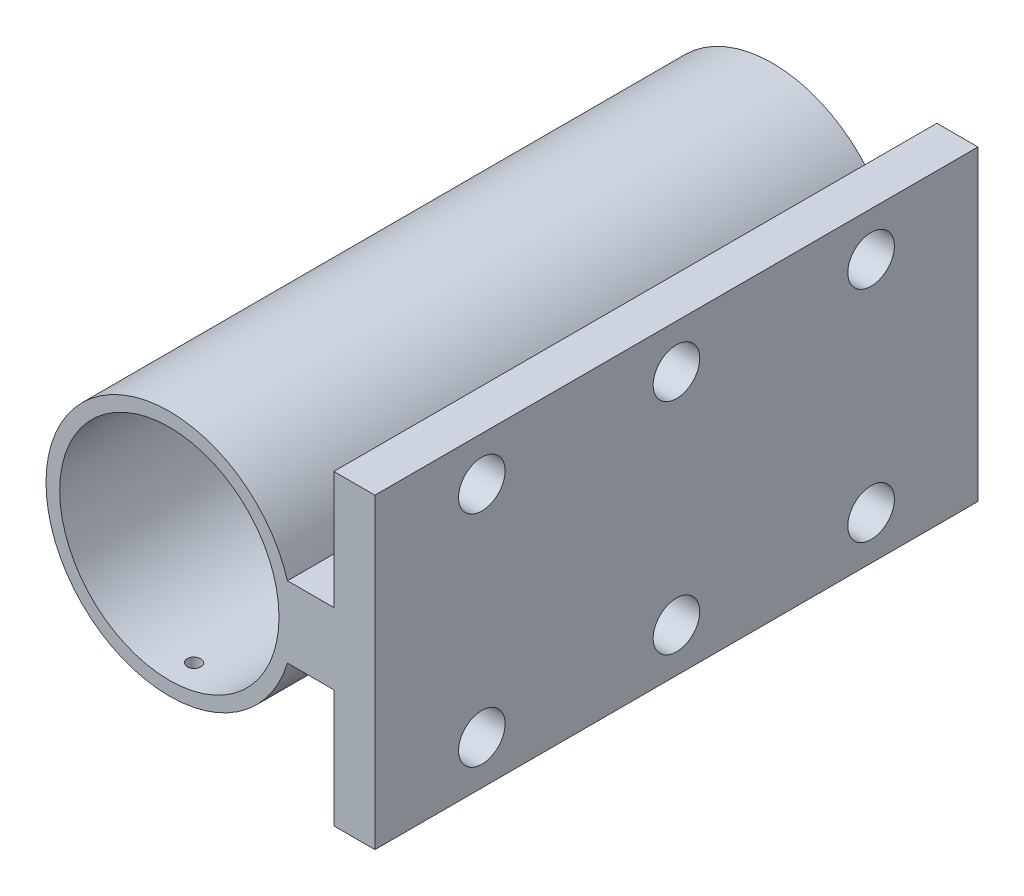
SolidWorks part; units mm, degrees
ref_plane "Front Plane" through (0, 0, 0) normal (0, 0, 1) x (1, 0, 0)
ref_plane "Top Plane" through (0, 0, 0) normal (0, 1, 0) x (1, 0, 0)
ref_plane "Right Plane" through (0, 0, 0) normal (1, 0, 0) x (0, 0, -1)
other "Configuration Table"
sketch "Sketch1" plane through (0, 0, 0) normal (0, 0, 1) x (1, 0, 0)
  line L0 (0, 0) -> (201.2265, 0) construction
  line L2 (75, 56) -> (60, 56)
  line L3 (75, 56) -> (75, -56)
  line L4 (75, -56) -> (60, -56)
  line L5 (60, 56) -> (60, 13)
  line L6 (75, 56) -> (60, -56) construction
  line L7 (75, -56) -> (60, 56) construction
  line L8 (43.0813, -13) -> (60, -13)
  line L10 (60, -13) -> (60, -56)
  line L11 (43.0813, 13) -> (60, 13)
  circle A0 centre (0, 0) radius 40
  arc A1 (43.0813, 13) -> (43.0813, -13) centre (0, 0) ccw
  point P5 (67.5, 0)
  dimension "D1" = 80
  dimension "D2" = 90
  dimension "D5" = 60
  dimension "D3" = 15
  dimension "D4" = 112
extrude "Boss-Extrude1" add sketch "Sketch1" along normal blind 220
sketch "Sketch2" plane through (75, 0, 0) normal (1, 0, 0) x (0, 0, -1)
  line L0 (0, -56) -> (0, 56) construction
  line L1 (-181, -40) -> (-39, -40) construction
  line L2 (-181, -40) -> (-181, 40) construction
  line L3 (-181, 40) -> (-39, 40) construction
  line L4 (-39, -40) -> (-39, 40) construction
  line L5 (-181, -40) -> (-39, 40) construction
  line L6 (-181, 40) -> (-39, -40) construction
  line L7 (-220, -56) -> (-220, 56) construction
  circle A0 centre (-181, -40) radius 8.5
  circle A1 centre (-181, 40) radius 8.5
  circle A2 centre (-110, 40) radius 8.5
  circle A3 centre (-110, -40) radius 8.5
  circle A4 centre (-39, -40) radius 8.5
  circle A5 centre (-39, 40) radius 8.5
  point P0 (-110, 0)
  point P7 (0, 0)
  dimension "D5" = 17
  dimension "D1" = 80
  dimension "D2" = 40
  dimension "D3" = 39
  dimension "D4" = 39
extrude "Cut-Extrude1" cut sketch "Sketch2" against normal up to next
sketch "Sketch3" plane through (0, 0, 0) normal (0, 1, 0) x (1, 0, 0)
  line L0 (40, 0) -> (-40, 0) construction
  line L1 (-45, -220) -> (43.0813, -220) construction
  circle A0 centre (0, -10) radius 2.5
  circle A1 centre (-0.9593, -210) radius 2.5
  dimension "D1" = 5
  dimension "D2" = 10
  dimension "D3" = 5
  dimension "D4" = 10
extrude "Cut-Extrude2" cut sketch "Sketch3" against normal up to next
